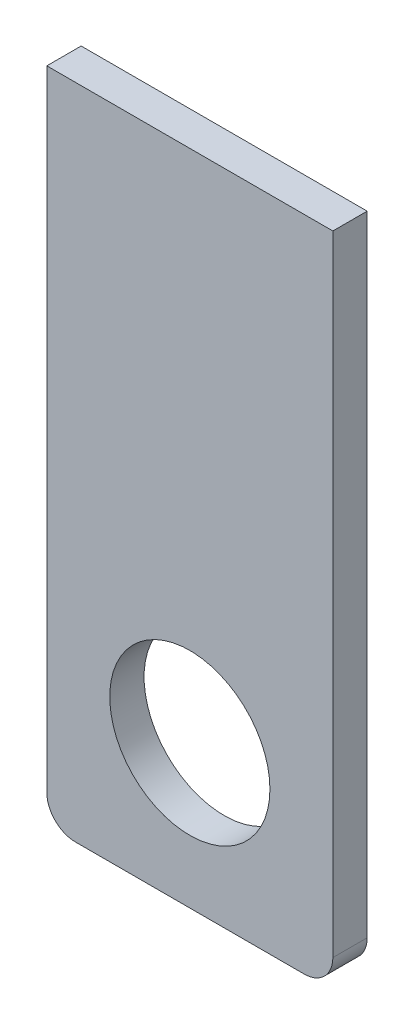
SolidWorks part; units mm, degrees
material "普通碳钢"
ref_plane "Front Plane" through (0, 0, 0) normal (0, 0, 1) x (1, 0, 0)
ref_plane "Top Plane" through (0, 0, 0) normal (0, 1, 0) x (1, 0, 0)
ref_plane "Right Plane" through (0, 0, 0) normal (1, 0, 0) x (0, 0, -1)
sketch "Sketch1" plane through (0, 0, 0) normal (0, 0, 1) x (1, 0, 0)
  line L1 (-25, 90) -> (25, 90)
  line L2 (-25, 90) -> (-25, -20)
  line L3 (-20, -25) -> (20, -25)
  line L4 (25, 90) -> (25, -20)
  circle A0 centre (0, 0) radius 14
  arc A1 (20, -25) -> (25, -20) centre (20, -20) ccw
  arc A2 (-25, -20) -> (-20, -25) centre (-20, -20) ccw
  point P9 (25, -25)
  dimension "D1" = 28
  dimension "D6" = 5
  dimension "D2" = 50
  dimension "D3" = 25
  dimension "D4" = 90
  dimension "D5" = 115
extrude "Boss-Extrude1" add sketch "Sketch1" along normal mid plane 6
